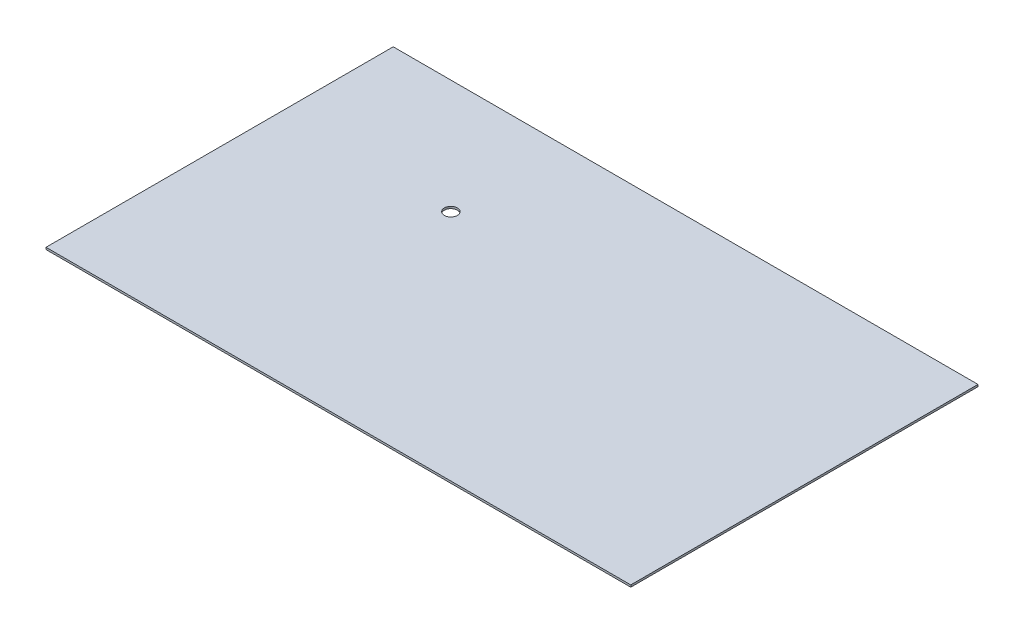
from build123d import *

# Parameters (mm, degrees)
SKETCH_1_W      = 2324
SKETCH_1_H      = 1380
SKETCH_1_R      = 26
EXTRUDE_1_DEPTH = 4


with BuildPart() as part:
    # 草图1 → 凸台-拉伸1 (new, symmetric)
    with BuildSketch(Plane(origin=(0, 0, 0), x_dir=(1, 0, 0), z_dir=(0, 1, 0))):
        Rectangle(SKETCH_1_W, SKETCH_1_H)
        with Locations(Location((-480, 237, 0), (0, 0, 270))):
            Circle(SKETCH_1_R, mode=Mode.SUBTRACT)
    extrude(amount=EXTRUDE_1_DEPTH, both=True)


solid = part.part
